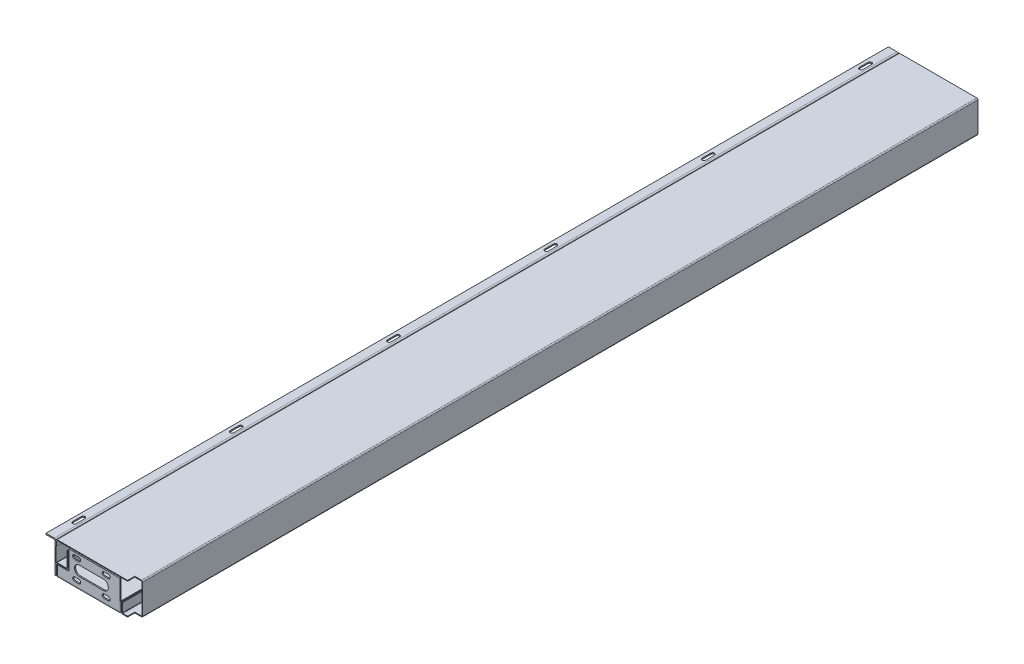
from build123d import *

# Parameters (mm, degrees)
EXTRUDE_1_DEPTH             = 1058
EXTRUDE_2_DEPTH             = 1058
EXTRUDE_2_2_DEPTH           = 1058
EXTRUDE_3_DEPTH             = 3
FILLET_1_R                  = 4
FILLET_2_R                  = 1
FILLET_3_R                  = 1
FILLET_4_R                  = 1
FILLET_5_R                  = 3
FILLET_6_R                  = 3
CUT_EXTRUDE_1_DEPTH         = 2127.935824138
CUT_EXTRUDE_3487_DEPTH      = 3
CUT_EXTRUDE_3708_DEPTH      = 1080.705515407
CUT_EXTRUDE_3708_DEPTH_BACK = 1080.705515407
SKETCH_6_W                  = 20
SKETCH_6_H                  = 18


with BuildPart() as part:
    # 草图1 → 凸台-拉伸1 (new, symmetric)
    with BuildSketch(Plane.XY):
        Polygon((-25, 0), (0, 0), (0, -80), (-3, -80), (-3, -3), (-25, -3), align=None)
    extrude(amount=EXTRUDE_1_DEPTH, both=True)

    # 圆角1
    fillet_1_edges = [part.edges().sort_by_distance(p)[0] for p in [
        (0, 0, 0),
    ]]
    fillet(fillet_1_edges, radius=FILLET_1_R)

    # 圆角2
    fillet_2_edges = [part.edges().sort_by_distance(p)[0] for p in [
        (-3, -3, 0),
    ]]
    fillet(fillet_2_edges, radius=FILLET_2_R)

    # 草图7 → Cut-Extrude 3487 (cut)
    with BuildSketch(Plane(origin=(0, 0, 0), x_dir=(1, 0, 0), z_dir=(0, 1, 0))):
        with BuildLine():
            Line((-17, 977), (-17, 999))
            ThreePointArc((-17, 999), (-12.5, 1003.5), (-8, 999))
            Line((-8, 999), (-8, 977))
            ThreePointArc((-8, 977), (-12.5, 972.5), (-17, 977))
        make_face()
        with BuildLine():
            Line((-17, 581.8), (-17, 603.8))
            ThreePointArc((-17, 603.8), (-12.5, 608.3), (-8, 603.8))
            Line((-8, 603.8), (-8, 581.8))
            ThreePointArc((-8, 581.8), (-12.5, 577.3), (-17, 581.8))
        make_face()
        with BuildLine():
            Line((-17, 186.6), (-17, 208.6))
            ThreePointArc((-17, 208.6), (-12.5, 213.1), (-8, 208.6))
            Line((-8, 208.6), (-8, 186.6))
            ThreePointArc((-8, 186.6), (-12.5, 182.1), (-17, 186.6))
        make_face()
        with BuildLine():
            Line((-17, -208.6), (-17, -186.6))
            ThreePointArc((-17, -186.6), (-12.5, -182.1), (-8, -186.6))
            Line((-8, -186.6), (-8, -208.6))
            ThreePointArc((-8, -208.6), (-12.5, -213.1), (-17, -208.6))
        make_face()
        with BuildLine():
            Line((-17, -603.8), (-17, -581.8))
            ThreePointArc((-17, -581.8), (-12.5, -577.3), (-8, -581.8))
            Line((-8, -581.8), (-8, -603.8))
            ThreePointArc((-8, -603.8), (-12.5, -608.3), (-17, -603.8))
        make_face()
        with BuildLine():
            Line((-17, -999), (-17, -977))
            ThreePointArc((-17, -977), (-12.5, -972.5), (-8, -977))
            Line((-8, -977), (-8, -999))
            ThreePointArc((-8, -999), (-12.5, -1003.5), (-17, -999))
        make_face()
    extrude(amount=-CUT_EXTRUDE_3487_DEPTH, mode=Mode.SUBTRACT)


with BuildPart() as body_2:
    # 草图2 → 凸台-拉伸2 (new, symmetric)
    with BuildSketch(Plane.XY):
        Polygon((0, 0), (0, -15), (2, -15), (2, -2), (198, -2), (198, -78), (167, -78), (167, -55), (165, -55), (165, -80), (200, -80), (200, 0), align=None)
    extrude(amount=EXTRUDE_2_DEPTH, both=True)

    # 圆角3
    fillet_3_edges = [body_2.edges().sort_by_distance(p)[0] for p in [
        (167, -78, 0),
        (198, -78, 0),
        (198, -2, 0),
        (2, -2, 0),
    ]]
    fillet(fillet_3_edges, radius=FILLET_3_R)

    # 圆角5
    fillet_5_edges = [body_2.edges().sort_by_distance(p)[0] for p in [
        (200, 0, 0),
        (200, -80, 0),
        (165, -80, 0),
        (0, 0, 0),
    ]]
    fillet(fillet_5_edges, radius=FILLET_5_R)

    # 草图6 → Cut-Extrude 3708 (cut, two sides: drawn at the far end of the back side and taken through both)
    with BuildSketch(Plane(origin=(0, 0, 0), x_dir=(1, 0, 0), z_dir=(0, 1, 0)).offset(-CUT_EXTRUDE_3708_DEPTH_BACK)):
        with Locations((190, -1049)):
            Rectangle(SKETCH_6_W, SKETCH_6_H)
    extrude(amount=CUT_EXTRUDE_3708_DEPTH + CUT_EXTRUDE_3708_DEPTH_BACK, mode=Mode.SUBTRACT)


with BuildPart() as body_3:
    # 草图2 → Extrude 2 2 (new, symmetric)
    with BuildSketch(Plane.XY):
        Polygon((0, -50), (0, -80), (163.5, -80), (163.5, -55), (161.5, -55), (161.5, -78), (2, -78), (2, -52), (30, -52), (30, -11), (28, -11), (28, -50), align=None)
    extrude(amount=EXTRUDE_2_2_DEPTH, both=True)

    # 圆角4
    fillet_4_edges = [body_3.edges().sort_by_distance(p)[0] for p in [
        (28, -50, 0),
        (2, -52, 0),
        (2, -78, 0),
        (161.5, -78, 0),
    ]]
    fillet(fillet_4_edges, radius=FILLET_4_R)

    # 圆角6
    fillet_6_edges = [body_3.edges().sort_by_distance(p)[0] for p in [
        (30, -52, 0),
        (163.5, -80, 0),
        (0, -80, 0),
        (0, -50, 0),
    ]]
    fillet(fillet_6_edges, radius=FILLET_6_R)


with BuildPart() as body_4:
    # 草图3 → 凸台-拉伸3 (new body)
    with BuildSketch(Plane.XY.offset(1058)):
        Polygon((160.5, -78), (160.5, -5), (33, -5), (33, -54), (4, -54), (4, -78), align=None)
    extrude(amount=-EXTRUDE_3_DEPTH)

    # 草图5 → 切除-拉伸1 (cut, through all)
    with BuildSketch(Plane.XY.offset(1058)):
        with BuildLine():
            Line((47, -11), (57, -11))
            ThreePointArc((57, -11), (62, -16), (57, -21))
            Line((57, -21), (47, -21))
            ThreePointArc((47, -21), (42, -16), (47, -11))
        make_face()
        with BuildLine():
            Line((47, -69), (57, -69))
            ThreePointArc((57, -69), (62, -64), (57, -59))
            Line((57, -59), (47, -59))
            ThreePointArc((47, -59), (42, -64), (47, -69))
        make_face()
        with BuildLine():
            Line((121, -11), (131, -11))
            ThreePointArc((131, -11), (136, -16), (131, -21))
            Line((131, -21), (121, -21))
            ThreePointArc((121, -21), (116, -16), (121, -11))
        make_face()
        with BuildLine():
            Line((121, -69), (131, -69))
            ThreePointArc((131, -69), (136, -64), (131, -59))
            Line((131, -59), (121, -59))
            ThreePointArc((121, -59), (116, -64), (121, -69))
        make_face()
        with BuildLine():
            Line((119, -52.5), (59, -52.5))
            ThreePointArc((59, -52.5), (46.5, -40), (59, -27.5))
            Line((59, -27.5), (119, -27.5))
            ThreePointArc((119, -27.5), (131.5, -40), (119, -52.5))
        make_face()
    extrude(amount=-CUT_EXTRUDE_1_DEPTH, mode=Mode.SUBTRACT)


with BuildPart() as body_5:
    # 镜向1: mirrored copy
    add(body_4.part.mirror(Plane.XY))


solid = Compound([part.part, body_2.part, body_3.part, body_4.part, body_5.part])
